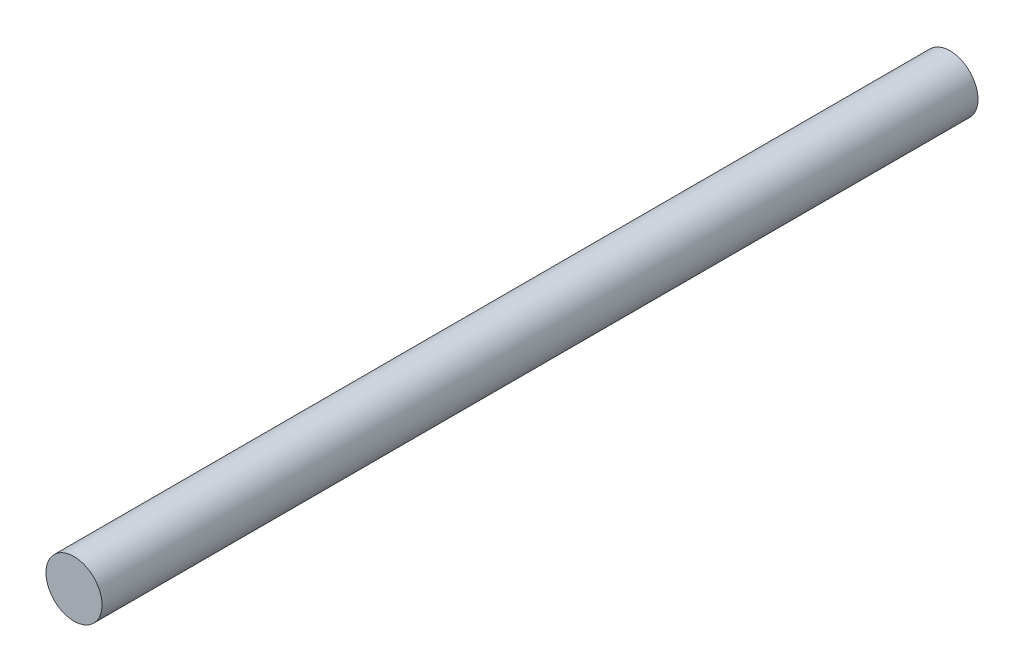
SolidWorks part; units mm, degrees
ref_plane "前视基准面" through (0, 0, 0) normal (0, 0, 1) x (1, 0, 0)
ref_plane "上视基准面" through (0, 0, 0) normal (0, 1, 0) x (1, 0, 0)
ref_plane "右视基准面" through (0, 0, 0) normal (1, 0, 0) x (0, 0, -1)
sketch "草图1" plane through (0, 0, 0) normal (0, 0, 1) x (1, 0, 0)
  circle A0 centre (0, 0) radius 8
  dimension "D1" = 16
extrude "凸台-拉伸1" add sketch "草图1" along normal blind 250
